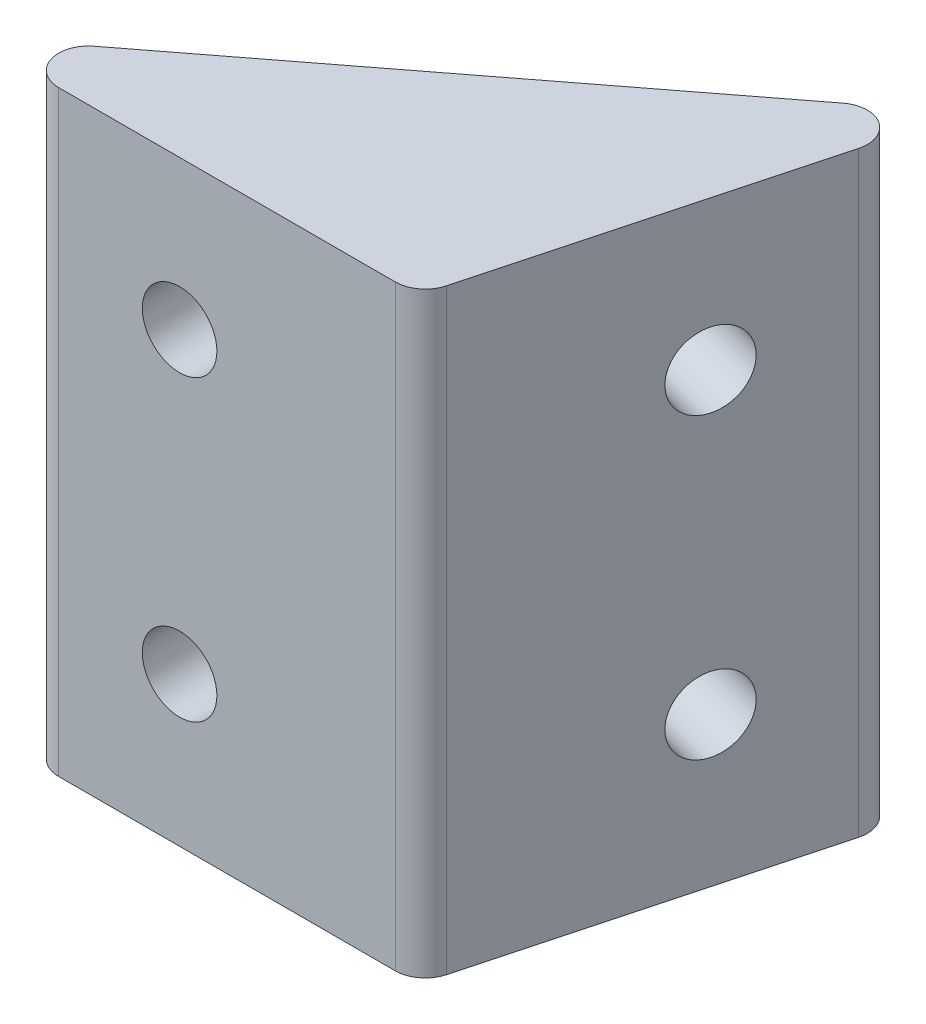
SolidWorks part; units mm, degrees
material "6061 合金"
ref_plane "前视基准面" through (0, 0, 0) normal (0, 0, 1) x (1, 0, 0)
ref_plane "上视基准面" through (0, 0, 0) normal (0, 1, 0) x (1, 0, 0)
ref_plane "右视基准面" through (0, 0, 0) normal (1, 0, 0) x (0, 0, -1)
other "Configuration Table"
sketch "草图1" plane through (0, 0, 0) normal (0, 1, 0) x (1, 0, 0)
  line L0 (0, 0) -> (15, 0)
  line L1 (15, 0) -> (18.8823, 14.4889)
  line L2 (18.8823, 14.4889) -> (0, 0)
  dimension "D1" = 105
  dimension "D2" = 15
extrude "凸台-拉伸1" add sketch "草图1" along normal blind 20
sketch "草图2" plane through (13.9952, 0, 3.75) normal (0.9659, 0, 0.2588) x (0.2588, 0, -0.9659)
  line L1 (3.8823, 20) -> (3.8823, 0) construction
  line L2 (3.8823, 0) -> (18.8823, 0) construction
  circle A2 centre (11.8823, 5) radius 1.6
  circle A4 centre (11.8823, 15) radius 1.6
  dimension "D2" = 3.2
  dimension "D1" = 8
  dimension "D3" = 10
  dimension "D4" = 5
hole_wizard "M3 螺纹孔1" positions "草图3" profile "草图4" tap size "M3" standard "GB"
sketch "草图3" plane through (13.9952, 0, 3.75) normal (0.9659, 0, 0.2588) x (0.2588, 0, -0.9659)
  point P0 (11.8823, 15)
  point P2 (11.8823, 5)
sketch "草图4" plane through (17.0706, 15, -7.7274) normal (0, 1, 0) x (0.2588, 0, -0.9659)
  line L0 (0, 0) -> (0, 7.5)
  line L1 (0, 7.5) -> (1.25, 6.7489)
  line L2 (1.25, 6.7489) -> (1.25, 0)
  line L5 (1.25, 0) -> (0, 0)
  line L10 (0, 7.5) -> (-1.25, 6.7489) construction
  line L11 (0, -6.35) -> (0, 107.95) construction
  dimension "螺纹孔钻头直径" = 2.5
  dimension "螺纹孔钻头深度" = 7.5
  dimension "导头角度" = 118
cosmetic thread "孔螺蚊线1" parameters "D1"=6, "D2"=3
cosmetic thread "孔螺蚊线2" parameters "D1"=6, "D2"=3
ref_plane "基准面1" through (9.4411, 0, -7.2444) normal (0.7934, 0, -0.6088) x (0, -1, 0)
mirror "镜向1" about plane through (9.4411, 0, -7.2444) normal (0.7934, 0, -0.6088) of "M3 螺纹孔1"
fillet "圆角1" radius 1 3 edges at (15, 10, 0) (0, 10, 0) (18.8823, 10, -14.4889)
